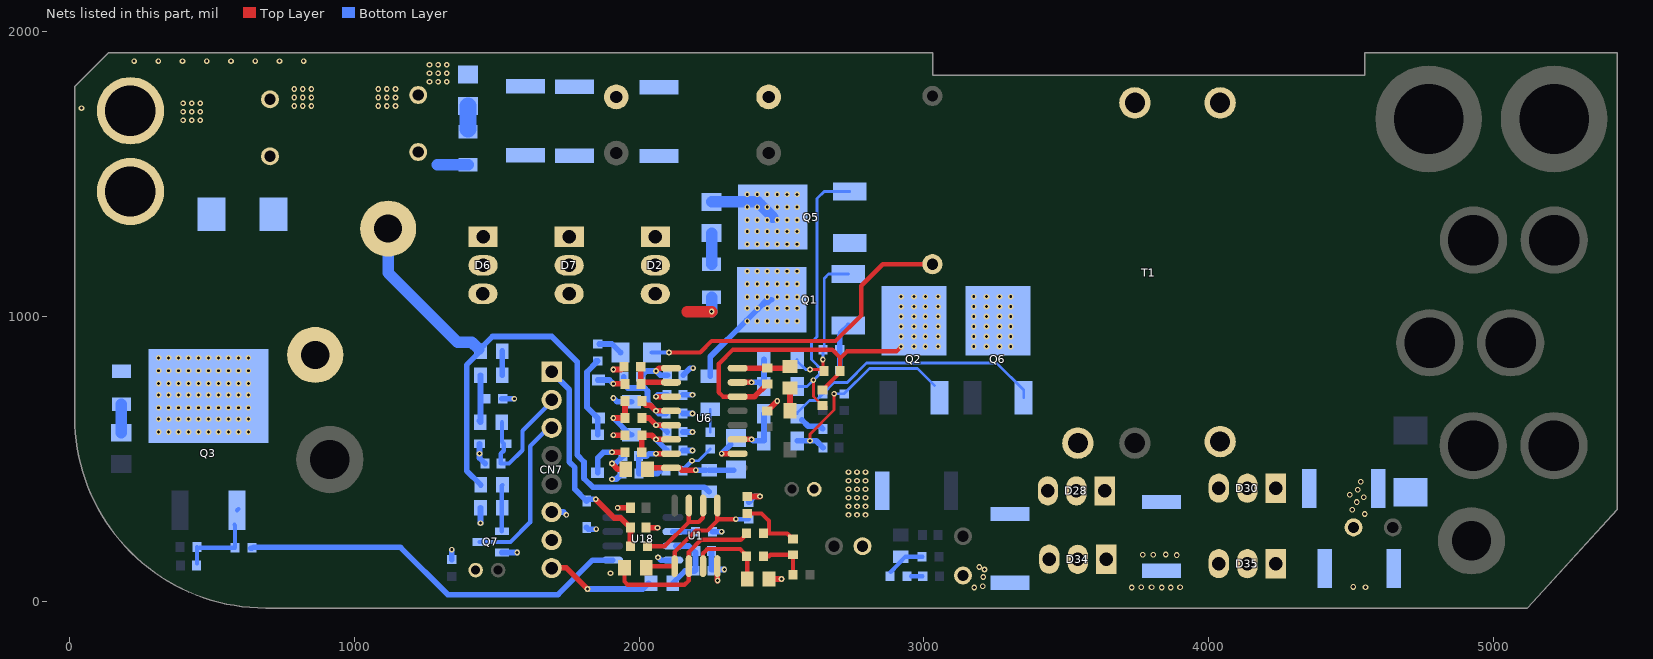
[diagram p0: the nets of this part, all layers, seen from the top]
# Altium PCB MISC84449.PcbDoc (part 2 of 3)
Units mil, origin at the board's own origin, x right, y up, seen from the top; angles counter-clockwise.
Board outline 5413.39 x 1948.82 mil, 4 copper layers (Top Layer, GND02, PWR03, Bottom Layer); 124 components, 66 nets, 298 pads, 442 vias.

## Via types
v1: diameter 20, hole 10, Top Layer to Bottom Layer, tented both sides, 231 vias
v2: diameter 20, hole 10, Top Layer to Bottom Layer, 187 vias
v3: diameter 20, hole 12, Top Layer to Bottom Layer, 24 vias

## Nets (pads, with @x,y where several pads share a name; then routed paths per layer and width w, separated by ;. In a path a pad name is that pad's centre, name@x,y a point inside that pad or via, vN(x,y) a via of type N, cw(c..) or ccw(c..) an arc to the next point about the centre after c; other vN are vias at no path point) (continued)
GND: C6.2 C7.1 C10.1 C11.2 C13.1 C14.1 C17.1 C18.1 C19.2 C21.1 C23.2 C24.2 C27.1 C72.1 C74.2 C75.2 C156.2 C169.2 CN7.6 D1.2 D4.2 D15.2 J6.2 Q7.2 R1.1 R4.1 R5.1 R7.2 R12.1 R15.2 R19.2 R28.1 R29.1 R30.1 R34.2 R186.2 R237.1 R271.1 R295.2 U1.4 U6.10 U18.4 | length 1573.3
  Top Layer w20: v1(1905,485) 1925,465 R5.1@1950.69,465 ; v1(1910,585) R12.1@1946.88,585 ; v1(1910,765) C10.1@1946.88,765 ; v1(1910,815) 1936.88,815 R1.1@1946.88,825 R1.1@1951.08,825 ; v1(1925,330) C24.2@1969.89,330 ; C7.1@2025,260 v1(2065,260) ; v1@2275,75 U1.4@2275,125 ; v1(2290,520) U6.10@2346.19,520 ; R186.2@2380,369.31 v1@2425,369.31 ; C17.1@2450,670.11 2450.11,670.11 v1(2485,705) ; R19.2@2456.08,80 v1(2500,80)
  Bottom Layer w20: R271.1@1343.01,148.02 v2(1343.01,182.99) ; D15.2@1440,555 v1(1440,520) 1440,504.89 C72.1@1459.89,485 ; v1(1443.92,276.08) R28.1@1443.92,330 ; Q7.2@1518.74,172.6 v1(1572.4,172.6) ; R29.1@1518.76,712.5 v1(1562.5,712.5) ; CN7.6@1672.49,315.01 1734.99,315.01 v1(1745,305) ; D1.2@1816,261 1822,255 v1@1848,255 ; D4.2@1855,778.27 1896.73,778.27 v1(1910,765) ; v1(1905,430) 1920,430 R4.1@1940,450 ; v1(1905,485) 1917.64,485 C11.2@1943.77,511.12 ; v1(1910,715) 1922.44,702.56 R15.2@1973.88,702.56 ; v2(2067,156) 2076.92,146.08 U18.4@2118.97,146.08 ; C18.1@2153.88,531.12 v1(2187.57,531.12) ; C14.1@2153.88,596.12 v1(2187.57,596.12) ; R7.2@2153.88,661.12 v1(2187.57,661.12) ; C19.2@2153.88,726.12 v1(2187.57,726.12) ; C13.1@2155,795 2180,820 v1(2190,820) ; C21.1@2254.48,179.36 2254.48,113.52 v2(2299.52,113.52) ; R237.1@2258.02,246.08 v2(2289.92,246.08) ; v1(2290,520) C27.1@2322,552 ; R34.2@2385,349.31 2405.69,370 v1(2425,370)
  other v1: 2276,75 1900,100 1850,255 2735,305 2765,305 2795,305 2735,335 2765,335 2795,335 2735,365 2765,365 2795,365 2735,395 2765,395 2795,395 2735,425 2765,425 2795,425 2735,455 2765,455 2795,455 400,1690 430,1690 460,1690 400,1720 430,1720 460,1720 42.92,1732.64 790,1740 820,1740 850,1740 1085,1740 1115,1740 1145,1740 400,1750 430,1750 460,1750 790,1770 820,1770 850,1770 1085,1770 1115,1770 1145,1770 790,1800 820,1800 850,1800 1085,1800 1115,1800 1145,1800 1265,1825 1295,1825 1325,1825 1265,1855 1295,1855 1325,1855 1265,1885 1295,1885 1325,1885 227.92,1897.64 312.92,1897.64 397.92,1897.64 482.92,1897.64 567.92,1897.64 652.92,1897.64 737.92,1897.64 822.92,1897.64
LLC_I: C15.1 C20.1 T1.3 | length 1174.2
  Top Layer w15: v1(2105,875) 2215,875 2255,915 2690,915 2780,1005 2780,1109 2855.73,1184.73 C20.1@3030,1184.73
  Bottom Layer w10: C15.1@2045,875 C15.1@2045.12,875
  Bottom Layer w15: C15.1@2045.12,875 v1(2105,875)
LO: R49.2 U18.5 | length 1383.7
  Bottom Layer w20: R49.2@637,188 R49.2@641,188 ; R49.2@647,191 1163,191 1329,25 1716,25 1837.08,146.08 U18.5@1907.75,146.08
NetC1_1: C1.1 C2.1 F1.1 R10.2 R33.2 R41.2 R43.2
  other v3: 3177,50 3730,50 3835,50 3866,50 3763,51 3799,51 3899,51 4550,51 4507,52 3207,54 3208,87 3212.71,113.27 3194,122 3887,164 3768,165 3805,165 3849,166 4547,308 4503,323 4519,350 4544,367 4495,376 4523,393 4533,421
NetC3_1: C3.1 C8.2 C73.1 Q1.2 Q5.2 R17.1 R25.2 R42.2 R46.2 | length 632.5
  Bottom Layer w15: Q1.2@2444.98,1039.76 Q1.2@2465.22,1060
  Bottom Layer w20: R17.1@2250,791.44 2250,860 2377.5,987.5 2417.5,1027.5 2450,1060 Q1.2@2465.22,1060
  Bottom Layer w40: C8.2@2255,1403.8 2380,1403.8 2415,1403.8 2416.2,1403.8 2425,1395 2442.5,1377.5 2465,1355 Q5.2@2470,1350
  other v2: 2380,985 2415,985 2450,985 2485,985 2520,985 2555,985 2380,1030 2415,1030 2450,1030 2485,1030 2520,1030 2555,1030 2380,1070 2415,1070 2450,1070 2485,1070 2520,1070 2555,1070 2380,1115 2415,1115 2450,1115 2485,1115 2520,1115 2555,1115 2380,1160 2415,1160 2450,1160 2485,1160 2520,1160 2555,1160 2380,1255 2415,1255 2450,1255 2485,1255 2520,1255 2555,1255 2380,1300 2415,1300 2450,1300 2485,1300 2520,1300 2555,1300 2380,1340 2415,1340 2450,1340 2485,1340 2520,1340 2555,1340 2380,1385 2415,1385 2450,1385 2485,1385 2520,1385 2555,1385 2380,1430 2415,1430 2450,1430 2485,1430 2520,1430 2555,1430
NetC4_1: C4.1 R2.2 | length 99.8
  Bottom Layer w40: C4.1@183,593.24 R2.2@183,693
NetC5_1: C5.1 Q3.1 R49.1 R98.2 | length 282.9
  Bottom Layer w15: C5.1@449,134 R98.2@449,192 ; R98.2@458,190 530,190 ; 517,190 530,190 ; Q3.1@580,270 582,268 R49.1@582,190 530,190 ; Q3.1@589,321 Q3.1@594,326
NetC6_1: C6.1 R31.2 | length 80
  Bottom Layer w60: R31.2@1400,1660 C6.1@1400,1740
NetC8_1: C8.1 R47.2 | length 108.6
  Bottom Layer w40: R47.2@2255,1185 C8.1@2255,1293.56
NetC9_1: C9.1 Q5.1 R22.1 R36.2 | length 970.7
  Top Layer w10: v2(2612,778) 2612,720.73 C9.1@2644.36,688.37
  Bottom Layer w10: R36.2@2555,755 2590,755 R22.1@2645,810 2605,850 2605,910 2625,930 2625,1415 2650.16,1440.16 Q5.1@2739.61,1440.16
NetC10_2: C10.2 R1.2 U6.2 | length 168.1
  Top Layer w20: R1.2@2006.19,825 C10.2@2006.19,765 2011.19,770 U6.2@2112.19,770
NetC11_1: C11.1 R4.2 R24.2 U6.7 | length 258.1
  Top Layer w20: v1(2060,520) U6.7@2112.19,520
  Bottom Layer w20: v1(2060,520) 2035,520 2026.12,511.12 C11.1@1998.88,511.12 1999.31,510.69 R4.2@1999.31,450 2065,450 2075,460
NetC12_1: C12.1 Q1.1 R20.2 R325.1 | length 520.3
  Top Layer w10: v1(2600,815) 2650,815 C12.1@2651,816 ; C12.1@2645.34,819.65 v1(2645.34,850.35)
  Bottom Layer w10: R20.2@2555,850 2555,845 2585,815 v1(2600,815) ; v1(2645.34,850.35) R325.1@2645.34,885 ; R325.1@2650,885 2650,1135 2665.16,1150.16 Q1.1@2734.82,1150.16
NetC13_2: C13.2 R6.2 U6.1 | length 164.5
  Top Layer w20: v1(2060,810) 2070,820 U6.1@2112.19,820
  Bottom Layer w20: R6.2@2006.19,790 2026.19,810 v1(2060,810) 2075,795 C13.2@2099.89,795
NetC14_2: C14.2 R8.2 U6.5 | length 161.2
  Top Layer w20: R8.2@2010,645 2035,645 v1(2060,620) U6.5@2112.19,620
  Bottom Layer w20: v1(2060,620) 2074.89,620 C14.2@2098.77,596.12
NetC15_2: C15.2 R14.1 | length 87.4
  Bottom Layer w20: R14.1@1860,905 1904.76,905 1934.82,874.94 C15.2@1934.88,874.88
NetC16_2: C16.2 R23.1 U6.16 | length 186.3
  Top Layer w20: U6.16@2346.19,820 C16.2@2450,820 2523.92,820 R23.1@2530,826.08
NetC18_2: C18.2 R12.2 R13.2 U6.6 | length 223.4
  Top Layer w20: R13.2@2009.65,525 2010,525.35 R12.2@2010,585 2045,585 v1(2060,570) U6.6@2112.19,570
  Bottom Layer w20: v1@2060,569.89 C18.2@2098.77,531.12
NetC19_1: C19.1 U6.3 | length 93.5
  Top Layer w20: v1(2060,720) U6.3@2112.19,720
  Bottom Layer w20: v1(2060,720) 2066.12,726.12 C19.1@2098.77,726.12
NetC21_2: C21.2 L12.2 R295.1 U18.3 | length 239.9
  Bottom Layer w20: L12.2@2117.96,64.36 2161.6,108 2195,108 2198,111 2198,173 2175,196 U18.3@2129,196
NetC22_1: C22.1 Q6.1 R37.1 R38.2 | length 1021.9
  Bottom Layer w10: R38.2@2555,660 2555,662 2599,706 2621,706 R37.1@2645,730 2685,770 2731,770 2799,838 3255,838 3350.16,742.84 Q6.1@3350.16,716.39
  Bottom Layer w20: R38.2@2572,638 2594,616 2636.01,616 C22.1@2645.08,606.92
NetC25_1: C25.1 Q2.1 R21.2 R302.1 | length 713
  Top Layer w10: v1(2600,565) 2600,588 2685,673 v1@2685,728
  Bottom Layer w10: v1(2685,730) R302.1@2720,730 2809,819 2977,819 Q2.1@3037,759
  Bottom Layer w20: R21.2@2555,565 v1(2600,565) 2622.01,565 C25.1@2646.08,540.92
NetC27_2: C27.2 R5.2 R44.1 U6.8 | length 294.7
  Top Layer w20: R5.2@2030,471 2031,470 U6.8@2112.19,470 2142,470 2150,462 v2(2199,462)
  Bottom Layer w20: v2(2199,462) R44.1@2234,462 ; R44.1@2245.92,462.07 C27.2@2332.93,462.07
NetC78_1: C78.1 R27.2 R186.1 | length 223
  Top Layer w15: R186.1@2380,310 2430,310 2456.08,283.92 2456.08,240 2520.11,240 C78.1@2540,220.11
NetC78_2: C78.2 R3.2 R338.1 | length 156.1
  Top Layer w15: 2456.08,160 2461.08,165 C78.2@2540,165 2540.34,164.65 R338.1@2540.34,95
NetD2_1: D2.1 D2.3 D6.1 D6.3 D7.1 D7.3 L4.2 Q3.2 R2.1 R47.1 | length 136.4
  Top Layer w40: 2168.56,1018.56 v1(2255,1018.56)
  Bottom Layer w40: v1(2255,1018.56) R47.1@2255,1068.56
  other v2: 314,596 349,596 384,596 419,596 454,596 489,596 524,596 559,596 594,596 629,596 314,641 349,641 384,641 419,641 454,641 489,641 524,641 559,641 594,641 629,641 314,681 349,681 384,681 419,681 454,681 489,681 524,681 559,681 594,681 629,681 314,726 349,726 384,726 419,726 454,726 489,726 524,726 559,726 594,726 629,726 314,766 349,766 384,766 419,766 454,766 489,766 524,766 559,766 594,766 629,766 314,811 349,811 384,811 419,811 454,811 489,811 524,811 559,811 594,811 629,811 314,856 349,856 384,856 419,856 454,856 489,856 524,856 559,856 594,856 629,856
NetD2_2: D2.2 R46.1
NetD3_1: D3.1 R13.1 | length 155.3
  Top Layer w20: v1(1905,525) R13.1@1950.34,525
  Bottom Layer w20: D3.1@1855,453.37 1855,505 1875,525 v1(1905,525)
NetD3_2: D3.2 D4.1 R14.2 | length 292.4
  Bottom Layer w20: R14.2@1848.5,844.5 R14.2@1849,845 ; R14.2@1850,846 R14.2@1849,845 ; R14.2@1852,841 1817.36,806.36 1817.36,682.64 1855,645 D3.2@1855,586.63 ; R14.2@1855,845 R14.2@1849,845
NetD5_1: D5.1 R23.2 | length 80
  Top Layer w20: D5.1@2530,670 R23.2@2530,750
NetD6_2: D6.2 R25.1
NetD7_2: D7.2 R42.1
NetD28_1: D28.1 D28.3 D34.1 D34.3 T1.8
NetD28_2: D28.2 R10.1
NetD30_1: D30.1 D30.3 D35.1 D35.3 T1.10
NetD30_2: D30.2 R33.1
NetD34_2: D34.2 R41.1
NetD35_2: D35.2 R43.1
NetQ7_1: Q7.1 R18.1 R28.2 | length 163.6
  Bottom Layer w15: Q7.1@1518.74,247.4 1518.74,330 1518.74,407.65 R18.1@1521.08,410
NetR3_1: R3.1 R19.1 U1.3 | length 296.6
  Top Layer w15: U1.3@2225,125 2225,170 2240,185 2355,185 2380,160 R19.1@2380,80
NetR6_1: R6.1 R7.1 R9.1 U6.4 | length 356.9
  Top Layer w20: R9.1@2010,705 2025,690 2040,690 v1(2060,670) U6.4@2112.19,670
  Bottom Layer w20: R6.1@1946.88,790 1946.88,763.12 1960,750 2020,750 2030,740 2030,700 v1(2060,670) 2068.88,661.12 R7.1@2094.57,661.12
NetR8_1: R8.1 R9.2 R15.1 | length 189
  Top Layer w20: v1(1910,645) 1950.69,645 R9.2@1950.69,705
  Bottom Layer w20: v1(1910,645) 1968.88,586.12 R15.1@1973.88,586.12
NetR11_1: R11.1 R34.1 U1.1 U1.5 | length 505.6
  Top Layer w15: R11.1@2030,125 U1.1@2125,125 2125,175 2200,250 2240,250 2275,285 2275,295 ; U1.5@2275,338 2275,295 ; v1(2340,290) 2280,290 2275,295
  Bottom Layer w15: v1(2340,290) R34.1@2385,290
NetR11_2: R11.2 R27.1 U1.2 | length 617.7
  Top Layer w15: R11.2@1948.92,120 1948.92,71.08 1960,60 2160,60 2175,75 U1.2@2175,125 2175,175 2217.5,217.5 2357.5,217.5 R27.1@2380,240
NetR16_1: R16.1 R17.2 | length 80
  Bottom Layer w10: R16.1@2250,595 R17.2@2250,675
NetR16_2: R16.2 R24.1 | length 130.3
  Bottom Layer w10: v1(2186.08,495) 2209.31,495 R16.2@2250,535.69
  Bottom Layer w15: R24.1@2151.08,460 2152.56,461.47 v1(2186.08,495)
NetR26_1: R26.1 R35.2 | length 85
  Bottom Layer w20: R35.2@1520,795 R26.1@1520,880
NetR29_2: R29.2 R35.1 R39.2 | length 171.1
  Bottom Layer w20: R39.2@1440,635 R39.2@1443.92,638.92 ; R39.2@1442.67,630 1443.92,631.24 R39.2@1443.92,638.92 ; R35.1@1443.92,795 1443.92,712.5 R39.2@1443.92,638.92
NetR32_1: R32.1 U1.6 U1.7 | length 337.8
  Top Layer w15: R32.1@2029.65,195 2090,195 2175,280 ; U1.7@2175,338 2175,280 ; U1.6@2225,338 2225,295 2210,280 2175,280
NetR40_1: R40.1 R53.2 R106.1 | length 134.3
  Bottom Layer w15: R106.1@2884,104.29 2935,158.29 R53.2@2995,158.29
NetR106_2: R106.2 R148.1 | length 40.7
  Bottom Layer w15: R106.2@2954.31,90 R148.1@2995,90
NetR237_2: R237.2 U18.2 | length 71.1
  Bottom Layer w20: U18.2@2118.97,246.08 R237.2@2190.08,246.08
PV+: F6.1 J6.1
PV-I: C7.2 CN7.1 D1.1 R32.2 | length 764
  Top Layer w20: v2@1848,359 1913,294 1935.89,294 C7.2@1969.89,260 1969.89,195.45 R32.2@1970.34,195
  Bottom Layer w20: CN7.1@1695,805 1755,745 1755,697 1755,491 1775,471 1775,395 D1.1@1816,354 ; D1.1@1816,353.33 1822.67,360 v2(1848,360)
PV-INT: CN7.3 Q7.3 | length 559.8
  Bottom Layer w15: Q7.3@1440,210 1549,210 1618,279 1618,546 CN7.3@1679,607
PV-OVP: C75.1 C169.1 F6.2 L4.1 R18.2 R26.2 R31.1 R44.2 | length 2501.2
  Bottom Layer w20: R26.2@1437.96,885.96 R26.2@1443.92,880 1395,831.08 1395,460 R18.2@1445,410 ; R26.2@1454,899 1486,931 1694,931 1783,842 1783,515 1807,491 1807,433 1838,402 1881,402 ; 1849,402 1881,402 ; R44.2@2245.92,385.99 2229.91,402 1881,402
  Bottom Layer w40: L4.1@1119.65,1309.62 1119.65,1154.35 1363,911 1413,911 R26.2@1438,886 ; 1291.44,1533.56 R31.1@1400,1533.56
PV-U: C72.2 CN7.2 D15.1 R39.1 | length 452.4
  Bottom Layer w15: R39.1@1518.76,630 1518.76,561.24 1525,555 1525,530 1515,520 C72.2@1515,485 1544,485 1591,532 1591,600 CN7.2@1688,697
PWM-H: CN7.7
PWM-L: CN7.8 L12.1 | length 376.9
  Top Layer w20: CN7.8@1695,119 1745,119 v2(1819,45)
  Bottom Layer w20: v2(1819,45) 2013,45 L12.1@2033,65
Q4G: R20.1 R36.1 U6.15 | length 193.6
  Top Layer w20: U6.15@2346.19,770 v1(2395,770)
  Bottom Layer w20: v1(2395,770) 2423.56,770 R36.1@2438.56,755 R20.1@2438.56,850
Q12G: R21.1 R38.1 U6.11 | length 189.4
  Top Layer w20: U6.11@2346.19,570 v1(2395,570)
  Bottom Layer w20: v1(2395,570) 2400,565 R21.1@2438.56,565 R38.1@2438.56,660
T1H: C9.2 C12.2 C16.1 Q1.3 Q2.2 Q5.3 Q6.2 R22.2 R325.2 T1.4 U6.14 | length 1274.7
  Top Layer w15: U6.14@2346.19,720 2295,720 2280,735 2280,835 2330,885 2678,885 2705.19,857.81 ; C9.2@2644.36,743.48 C12.2@2704,803.12 ; C12.2@2705.19,810.08 2705.19,833 ; 2705.19,843 2705.19,833 ; v2@2918,893 2904,879 2730,879 2705.19,854.19 2705.19,833
  Top Layer w20: U6.14@2346.19,720 2405.11,720 C16.1@2450,764.89
  Bottom Layer w20: R22.2@2704.31,810 R325.2@2704.31,870 ; R325.2@2704.65,875 R325.2@2704.65,885 2704.65,934.33 ; Q1.3@2709.31,944.33 Q1.3@2734.82,969.84
  other v2: 2920,896 2965,896 3005,896 3050,896 3175,896 3220,896 3265,896 3305,896 2920,931 2965,931 3005,931 3050,931 3175,931 3220,931 3265,931 3305,931 2920,966 2965,966 3005,966 3050,966 3175,966 3220,966 3265,966 3305,966 2920,1001 2965,1001 3005,1001 3050,1001 3175,1001 3220,1001 3265,1001 3305,1001 2920,1036 2965,1036 3005,1036 3050,1036 3175,1036 3220,1036 3265,1036 3305,1036 2920,1071 2965,1071 3005,1071 3050,1071 3175,1071 3220,1071 3265,1071 3305,1071
pads on no net: U6.9 U6.13 U18.6 U18.7 U18.8

## Polygon pours and split planes (outlines as drawn)
LLC_I on Top Layer "BottomLayer-No Net" (solid, remove dead copper, pour order 1002): 2915,1316 2915,1190 2939,1166 2957,1148 2981,1148 3333,1148 3388,1203 3392,1207 3392,1242 3392,1348 3441,1397 3561,1517 3669,1517 3984,1517 4057,1590 4130,1663 4130,1719 4130,1781 4115,1796 4100,1811 4061,1811 3991,1811 3936,1756 3856,1676 3732,1676 3329,1676 3060,1407 3049,1396 2995,1396 2967,1396 2942,1371 2915,1344 2915,1316
NetD30_1 on Top Layer "BottomLayer-No Net" (solid, remove dead copper, pour order 1001): 3936,579 3936,82 3953,65 3965,53 3988,53 4297,53 4313,69 4315,71 4315,83 4315,484 4196,603 4164,635 4083,635 3980,635 3948,603 3936,591 3936,579
NetD28_1 on Top Layer "BottomLayer-No Net" (solid, remove dead copper, pour order 1000): 3332,427 3332,420 3332,99 3359,72 3372,59 3414,59 3692,59 3716,83 3727,94 3727,120 3727,449 3671,505 3661,515 3661,546 3661,611 3645,627 3623,649 3585,649 3450,649 3410,609 3332,531 3332,429
NetC1_1 on Top Layer "BottomLayer-No Net" (solid, remove dead copper, pour order 1001): 3104,102.76 3104,42.89 3126.24,20.94 3156.56,-9 3229.34,-9 4576.76,-9 4596.98,10.96 4599,12.95 4599,30.91 4599,52.87 4578.78,72.82 4565.64,85.8 4565.64,196.56 4565.64,442.03 4560.59,447.02 4553.51,454 4519.15,454 4427.16,454 4409.98,437.04 4384.71,412.09 4384.71,341.24 4384.71,87.79 4357.41,60.85 4330.12,33.91 4257.34,33.91 3943.99,33.91 3909.62,67.83 3902.55,74.82 3873.23,74.82 3727.67,74.82 3712.51,59.85 3699.37,46.88 3681.18,46.88 3248.55,46.88 3224.29,70.83 3224.29,106.75 3224.29,127.7 3217.21,134.69 3212.16,139.68 3200.03,139.68 3128.26,139.68 3109.05,120.72 3104,115.73 3104,103.76
B+ on Top Layer "BottomLayer-No Net" (solid, remove dead copper, pour order 1000): 4571,1766.66 4571,607.38 4590,587.82 4600,577.52 4675,577.52 4771,577.52 4786,562.08 4800,547.66 4800,519.87 4800,478.68 4841,436.47 4857,420 4938,420 5002,420 5039,458.09 5062,481.77 5062,607.38 5062,633.12 4938,760.78 4904,795.79 4904,921.39 4904,1032.59 5018,1149.96 5053,1185.99 5053,1302.33 5053,1350.72 5004,1401.17 4976,1430 4976,1683.27 4976,1796.52 4911,1863.44 4892,1883 4813,1883 4646,1883 4584,1819.17 4570,1804.75 4570,1769.75
NetD2_1 on Top Layer "BottomLayer-No Net" (solid, remove dead copper, pour order 1000): 785,1086 747,1086 694,1086 643,1035 579,971 384,971 168,971 126,929 94,897 94,797 94,464 180,378 251,307 533,307 546,307 646,407 695,456 695,564 695,589 738,632 787,681 888,681 1364,681 1565,882 1602,919 1996,919 2135,919 2172,956 2191,975 2191,1007 2191,1404 2157,1438 2149,1446 2069,1446 1397,1446 1358,1407 1329,1378 1329,1343 1329,1190 1249,1110 1225,1086 785,1086
NetC3_1 on Top Layer "BOTTOM-No Net" (solid, remove dead copper, pour order 1000): 2575,1470 2585,1460 2585,965 2575,955 2345,955 2335,965 2335,1460 2345,1470
T1H on Top Layer "BOTTOM-No Net" (solid, remove dead copper, pour order 1001): 2865,1107 3380,1107 3395,1092 3395,872 3385,862 2850,862 2840,872 2840,1102 2845,1107 2865,1107
GND on Top Layer "BOTTOM-No Net" (solid, remove dead copper, pour order 1004): 1440,1580 1440,1910 1420,1930 100,1930 30,1860 15,1845 15,1085 35,1065 80,1065 485,1065 580,1160 600,1180 985,1180 1185,1180 1245,1240 1245,1385 1245,1495 1290,1540 1305,1555 1345,1555 1415,1555 1440,1580
+12V on Top Layer "BOTTOM-No Net" (solid, remove dead copper, pour order 1010): 2600,150 2590,160 2590,245 2550,285 2505,285 2485,305 2485,320 2400,405 2400,625 2405,630 2475,630 2525,580 2560,580 2570,570 2570,375 2730,215 2730,155 2725,150
BAT- on Top Layer "BOTTOM-No Net" (solid, remove dead copper, pour order 1011): 2854.67,810 3282.12,810 3302,786.87 3302,249.05 3302,214.35 3287.09,197 3053.49,197 3038.57,214.35 3038.57,474.58 3028.63,486.15 2998.81,520.85 2864.61,520.85 2814.91,520.85 2800,538.2 2800,792.65 2814.91,810 2854.67,810
GND on Top Layer "BOTTOM-No Net" (solid, remove dead copper, pour order 1012): 2625,490 2865,490 2875,480 2875,180 2865,170 2760,170 2750,180 2750,240 2720,270 2595,395 2595,470 2595,480 2600,485 2605,490 2625,490